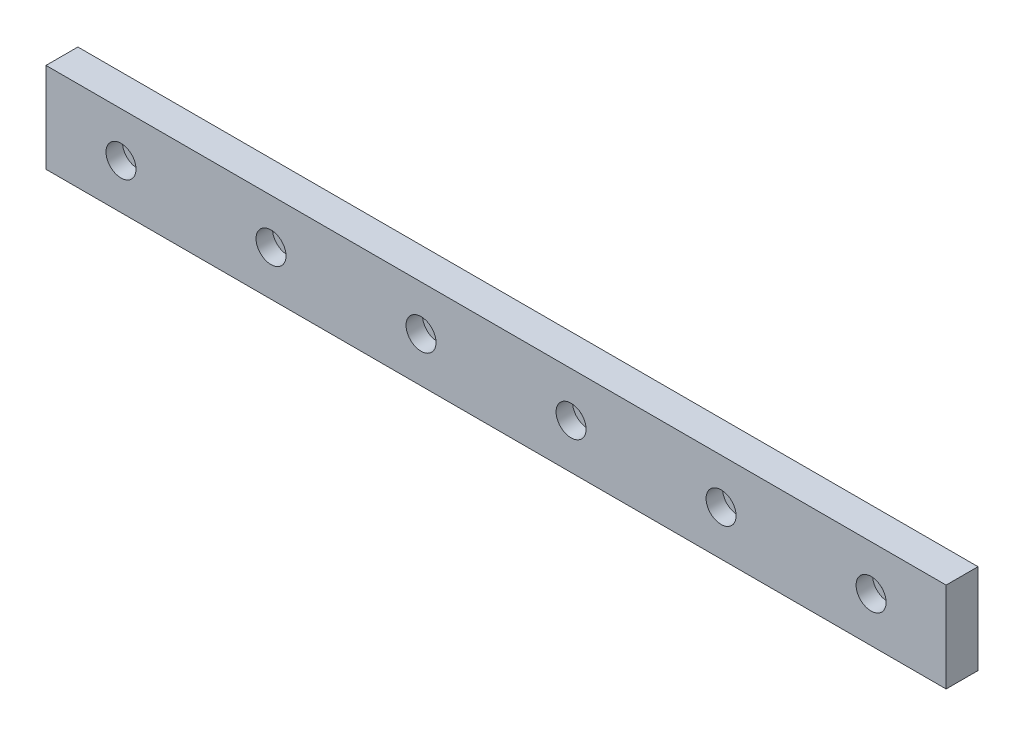
SolidWorks part; units mm, degrees
material "6061"
ref_plane "Front Plane" through (0, 0, 0) normal (0, 0, 1) x (1, 0, 0)
ref_plane "Top Plane" through (0, 0, 0) normal (0, 1, 0) x (1, 0, 0)
ref_plane "Right Plane" through (0, 0, 0) normal (1, 0, 0) x (0, 0, -1)
sketch "Sketch1" plane through (0, 0, 0) normal (0, 0, 1) x (1, 0, 0)
  line L1 (-120, 12) -> (120, 12)
  line L2 (-120, 12) -> (-120, -12)
  line L3 (-120, -12) -> (120, -12)
  line L4 (120, 12) -> (120, -12)
  line L5 (-120, 12) -> (120, -12) construction
  line L6 (-120, -12) -> (120, 12) construction
  point P0 (0, 0)
  dimension "D1" = 24
  dimension "D2" = 240
extrude "Boss-Extrude1" add sketch "Sketch1" along normal blind 8.5
hole_wizard "CBORE for M4 Hex Socket Head Cap Screw1" positions "Sketch3" profile "Sketch2" counterbore size "M4" standard "Iso" end condition through all
sketch "Sketch3" plane through (0, 0, 8.5) normal (0, 0, 1) x (1, 0, 0)
  line L0 (-120, 0) -> (-151.984, 0) construction
  line L1 (-120, 12) -> (-120, -12) construction
  point P0 (-100, 0)
  dimension "D1" = 20
sketch "Sketch2" plane through (-100, 0, 8.5) normal (1, 0, 0) x (0, -1, 0)
  line L0 (0, 0) -> (0, 8.5)
  line L1 (0, 8.5) -> (2.25, 8.5)
  line L3 (2.25, 8.5) -> (2.25, 4.4)
  line L4 (2.25, 4.4) -> (4, 4.4)
  line L5 (4, 4.4) -> (4, 0)
  line L7 (4, 0) -> (0, 0)
  line L11 (0, -6.35) -> (0, 107.95) construction
  dimension "通孔孔直径" = 4.5
  dimension "通孔孔深度" = 8.5
  dimension "柱形沉头孔直径" = 8
  dimension "柱形沉头孔深度" = 4.4
pattern_linear "LPattern1" count 6 spacing 40 along (1, 0, 0) of "CBORE for M4 Hex Socket Head Cap Screw1"
